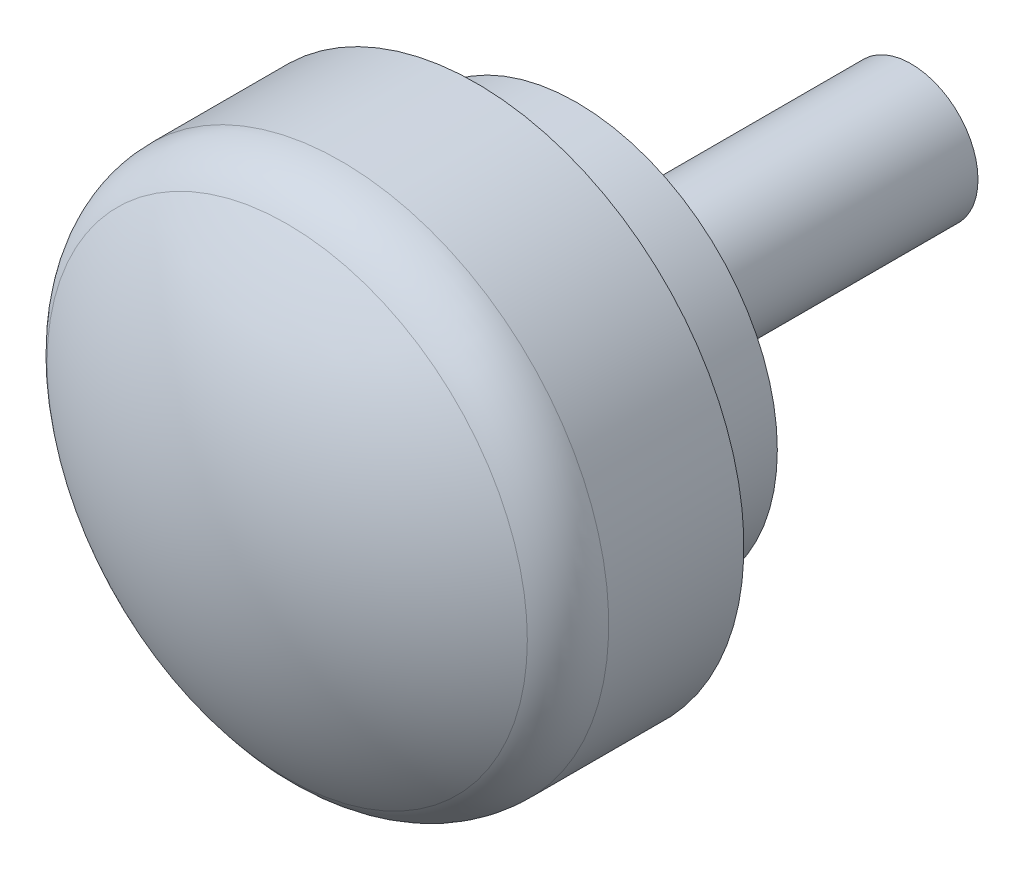
from build123d import *

# Parameters (mm, degrees)
SKETCH1_R           = 2
BOSS_EXTRUDE1_DEPTH = 10
SKETCH2_R           = 8
BOSS_EXTRUDE2_DEPTH = 8
SKETCH3_R           = 8
SKETCH3_R_2         = 6
CUT_EXTRUDE1_DEPTH  = 3
DOME1_FACE_RADIUS   = 8
DOME1_HEIGHT        = 3
FILLET1_R           = 2


with BuildPart() as part:
    # Sketch1 → Boss-Extrude1 (new body)
    with BuildSketch(Plane.XY):
        Circle(SKETCH1_R)
    extrude(amount=BOSS_EXTRUDE1_DEPTH)

    # Sketch2 → Boss-Extrude2 (add)
    with BuildSketch(Plane.XY.offset(10)):
        Circle(SKETCH2_R)
    extrude(amount=BOSS_EXTRUDE2_DEPTH)

    # Sketch3 → Cut-Extrude1 (cut)
    with BuildSketch(Plane(origin=(0, 0, 10), x_dir=(-1, 0, 0), z_dir=(0, 0, -1))):
        Circle(SKETCH3_R)
        Circle(SKETCH3_R_2, mode=Mode.SUBTRACT)
    extrude(amount=-CUT_EXTRUDE1_DEPTH, mode=Mode.SUBTRACT)

    # Dome1: a dome of height H over a round flat face of radius A is a cap of a sphere of radius (A * A + H * H) / (2 * H)
    dome1_r = (DOME1_FACE_RADIUS * DOME1_FACE_RADIUS + DOME1_HEIGHT * DOME1_HEIGHT) / (2 * DOME1_HEIGHT)
    dome1_base = Plane((0, 0, 18), z_dir=(0, 0, 1))
    with Locations(dome1_base.offset(DOME1_HEIGHT - dome1_r)):
        dome1_ball = Sphere(dome1_r, mode=Mode.PRIVATE)
    add(split(dome1_ball, bisect_by=dome1_base, keep=Keep.TOP, mode=Mode.PRIVATE))

    # Fillet1
    fillet1_edges = [part.edges().sort_by_distance(p)[0] for p in [
        (-8, 0, 18),
    ]]
    fillet(fillet1_edges, radius=FILLET1_R)


solid = part.part
